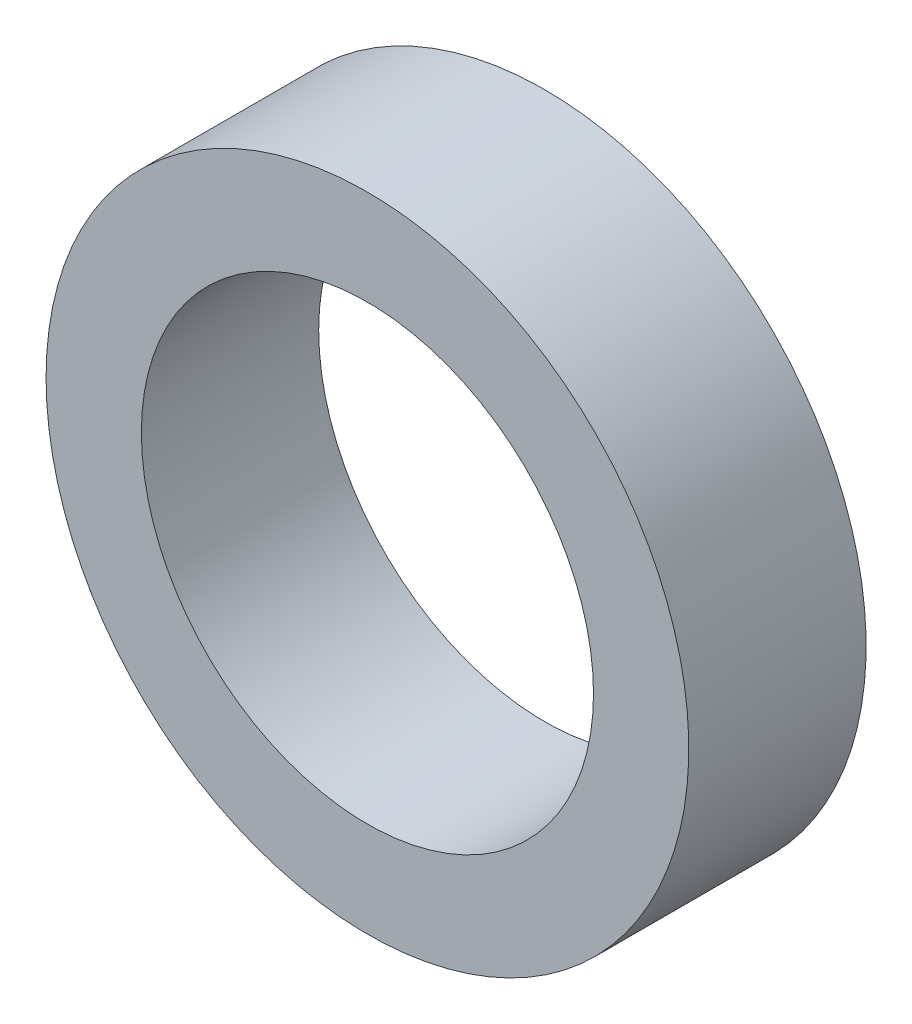
from build123d import *

# Parameters (mm, degrees)
SKETCH1_W = 2.15
SKETCH1_H = 4


with BuildPart() as part:
    # Sketch1 → Revolve1 (revolve)
    with BuildSketch(Plane.XZ, mode=Mode.PRIVATE) as revolve1_sk:
        with Locations((6.175, 0)):
            Rectangle(SKETCH1_W, SKETCH1_H)
    revolve(revolve1_sk.sketch.rotate(Axis((0, 0, 2), (0, 0, -1)), 180), axis=Axis((0, 0, 2), (0, 0, -1)))


solid = part.part
